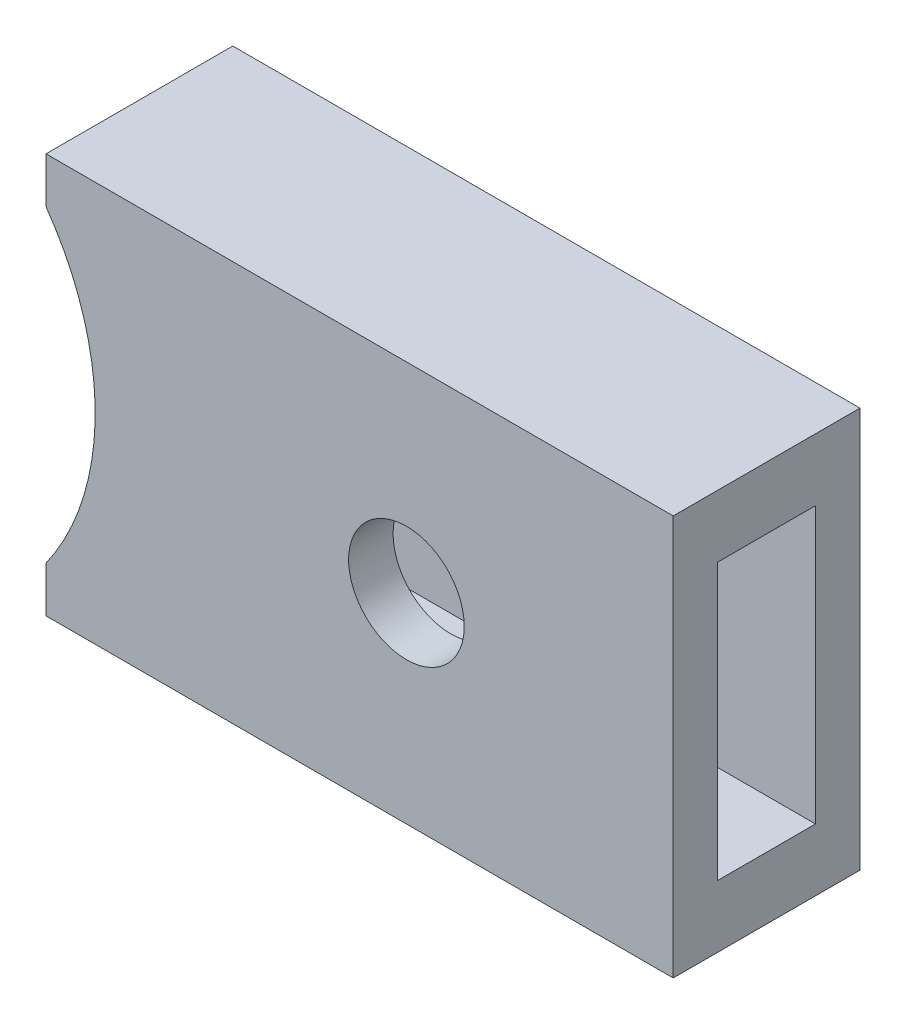
SolidWorks part; units mm, degrees
material "AISI 1045 钢，冷拔"
ref_plane "前视基准面" through (0, 0, 0) normal (0, 0, 1) x (1, 0, 0)
ref_plane "上视基准面" through (0, 0, 0) normal (0, 1, 0) x (1, 0, 0)
ref_plane "右视基准面" through (0, 0, 0) normal (1, 0, 0) x (0, 0, -1)
sketch "草图1" plane through (0, 0, 0) normal (0, 0, 1) x (1, 0, 0)
  line L0 (95, 22.5) -> (95, -22.5)
  line L1 (0, 0) -> (232.642, 0) construction
  line L2 (24.4737, 22.5) -> (95, 22.5)
  line L3 (24.4737, -22.5) -> (95, -22.5)
  line L4 (24.4737, 22.5) -> (24.4737, 17.3505)
  line L5 (24.4737, -17.3505) -> (24.4737, -22.5)
  arc A0 (24.4737, 17.3505) -> (24.4737, -17.3505) centre (0, 0) cw
  point P2 (70, 0)
  dimension "D1" = 95
  dimension "D2" = 25
  dimension "D3" = 45
extrude "凸台-拉伸1" add sketch "草图1" along normal mid plane 21
sketch "草图2" plane through (95, 0, 0) normal (1, 0, 0) x (0, 0, -1)
  line L0 (-24.4364, 0) -> (19.9033, 0) construction
  line L1 (-5.5, 15.5) -> (5.5, 15.5)
  line L2 (-5.5, -15.5) -> (5.5, -15.5)
  line L3 (0, 27.0925) -> (0, -28.5091) construction
  line L4 (-5.5, 15.5) -> (-5.5, -15.5)
  line L5 (5.5, 15.5) -> (5.5, -15.5)
  dimension "D1" = 31
  dimension "D2" = 11
extrude "切除-拉伸1" cut sketch "草图2" against normal through all
sketch "草图3" plane through (0, 0, 10.5) normal (0, 0, 1) x (1, 0, 0)
  line L0 (24.4737, -22.5) -> (95, -22.5) construction
  line L1 (95, -22.5) -> (95, 22.5) construction
  line L2 (95, 22.5) -> (24.4737, 22.5) construction
  line L3 (24.4737, -22.5) -> (95, -22.5)
  line L4 (95, -22.5) -> (95, 22.5)
  line L5 (95, 22.5) -> (24.4737, 22.5)
  line L6 (53.4102, 0) -> (79.9312, 0) construction
  line L7 (65, -10.6585) -> (65, 10.4545) construction
  line L8 (56.4723, 10) -> (83.5011, 10) construction
  line L9 (56.4723, -10) -> (83.5011, -10) construction
  line L10 (59.1414, 10) -> (53.4102, 0)
  line L11 (53.4102, 0) -> (59.1414, -10)
  line L12 (59.1414, -10) -> (70.8586, -10)
  line L13 (70.8586, -10) -> (76.5898, 0)
  line L14 (76.5898, 0) -> (70.8586, 10)
  line L15 (70.8586, 10) -> (59.1414, 10)
  circle A0 centre (65, 0) radius 6.5
  point P0 (65, 0)
  point P16 (53.45, 0)
  point P17 (76.55, 0)
  point P18 (73.7242, -5)
  point P19 (59.1414, 10)
  point P20 (70.8586, 10)
  point P21 (70.8586, -10)
  point P22 (59.1414, -10)
  dimension "D2" = 20
  dimension "D1" = 30
  dimension "D3" = 23.1
  dimension "D4" = 12.5
  dimension "D5" = 12.5
  dimension "D6" = 10.0554
  dimension "D7" = 11.5259
  dimension "D8" = 11.5259
  dimension "D9" = 10.0554
extrude "切除-拉伸2" cut sketch "草图3" against normal up to next contours A0
sketch "草图4" plane through (0, 0, -10.5) normal (0, 0, -1) x (-1, 0, 0)
  line L0 (-82.0533, 0) -> (-57.7577, 0) construction
  line L1 (-65, 11.7751) -> (-65, -12.5015) construction
  line L4 (-70.7795, 10) -> (-76.55, 0)
  line L5 (-76.55, 0) -> (-70.7795, -10)
  line L10 (-59.2205, 10) -> (-53.45, 0)
  line L11 (-53.45, 0) -> (-59.2205, -10)
  line L12 (-70.7795, 10) -> (-59.2205, 10)
  line L13 (-70.7795, -10) -> (-59.2205, -10)
  line L14 (-95, -22.5) -> (-95, 22.5) construction
  line L15 (-95, 22.5) -> (-24.4737, 22.5) construction
  line L16 (-24.4737, -22.5) -> (-95, -22.5) construction
  circle A2 centre (-65, 0) radius 6.5
  point P8 (-76.55, 0)
  point P9 (-53.45, 0)
  point P15 (-70.7795, 10)
  point P16 (-59.2205, 10)
  point P17 (-59.2205, -10)
  point P18 (-70.7795, -10)
  dimension "D1" = 23.1
  dimension "D2" = 30
  dimension "D3" = 11.5455
  dimension "D4" = 12.5
  dimension "D5" = 12.5
  dimension "D6" = 11.5455
  dimension "D7" = 10.0039
  dimension "D8" = 11.5455
  dimension "D9" = 11.5455
extrude "切除-拉伸5" cut sketch "草图4" against normal up to next contours L5 L13 L11 L10 L12 L4 A2 | A2
